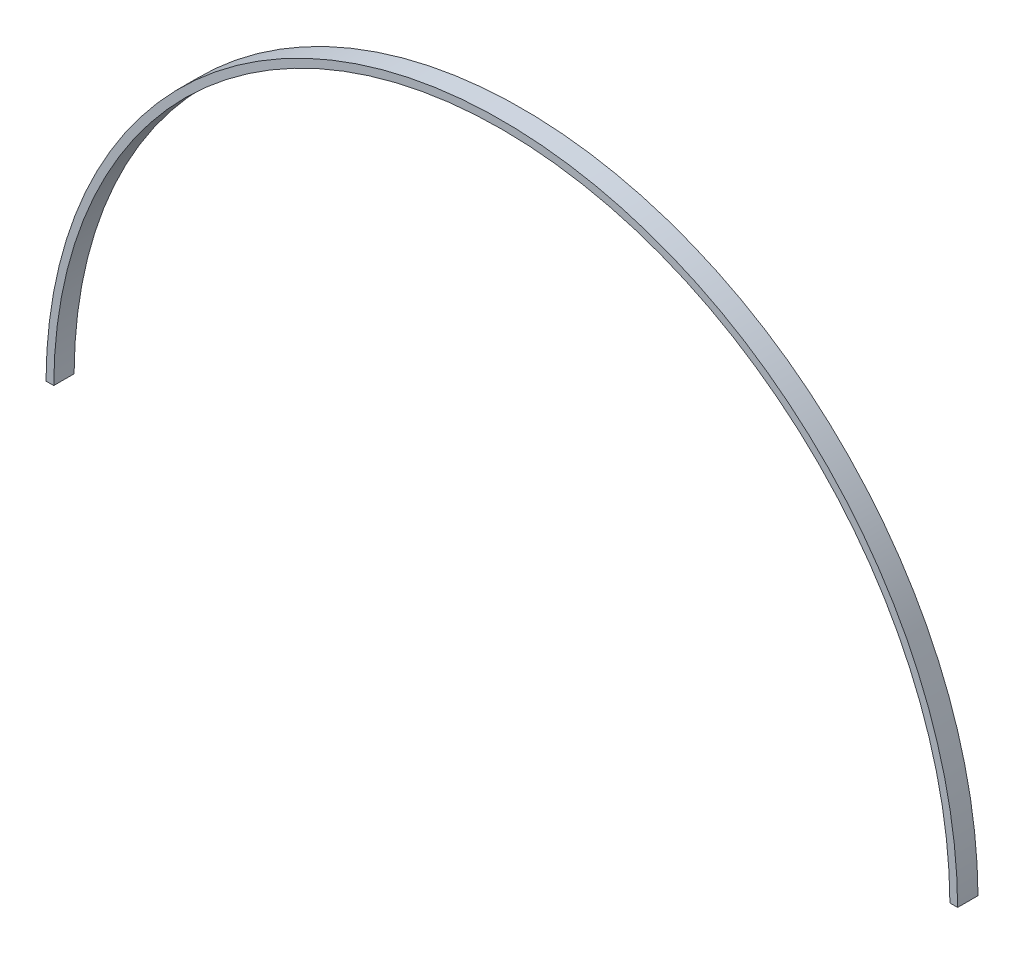
from build123d import *

# Parameters (mm, degrees)
EXTRUDE_1_DEPTH = 5


with BuildPart() as part:
    # 草图1 → 凸台-拉伸1 (new, symmetric)
    with BuildSketch(Plane.XY):
        with BuildLine():
            Line((-3.997767846, 1), (-0.197729325, 1))
            ThreePointArc((-0.197729325, 1), (220, 220.2), (440.197729325, 1))
            Line((440.197729325, 1), (443.997767846, 1))
            ThreePointArc((443.997767846, 1), (220, 224), (-3.997767846, 1))
        make_face()
    extrude(amount=EXTRUDE_1_DEPTH, both=True)


solid = part.part
